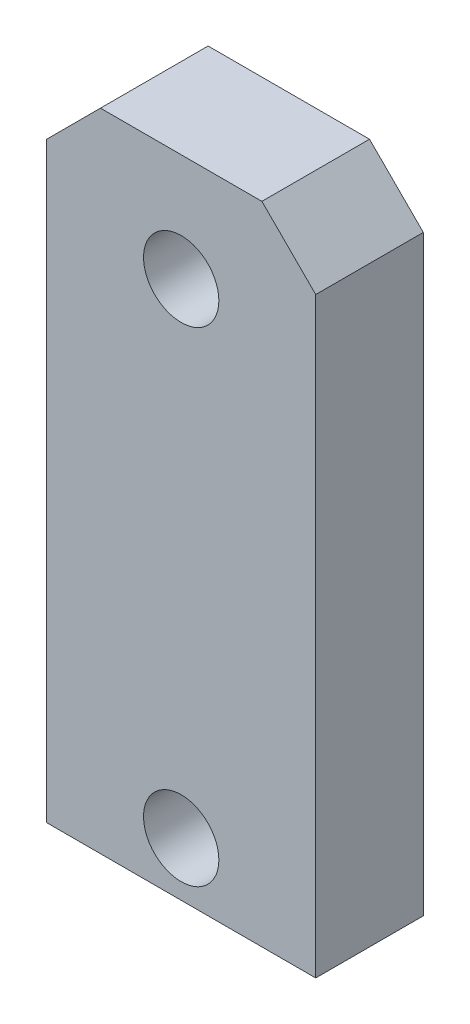
from build123d import *

# Parameters (mm, degrees)
SKETCH1_W           = 25
SKETCH1_H           = 60
BOSS_EXTRUDE1_DEPTH = 10
SKETCH2_R           = 3.5
CUT_EXTRUDE1_DEPTH  = 10
CHAMFER1_SIZE       = 5


with BuildPart() as part:
    # Sketch1 → Boss-Extrude1 (new body)
    with BuildSketch(Plane.XY):
        Rectangle(SKETCH1_W, SKETCH1_H)
    extrude(amount=BOSS_EXTRUDE1_DEPTH)

    # Sketch2 → Cut-Extrude1 (cut)
    with BuildSketch(Plane.XY.offset(10)):
        with Locations((0, 20)):
            Circle(SKETCH2_R)
        with Locations((0, -25)):
            Circle(SKETCH2_R)
    extrude(amount=-CUT_EXTRUDE1_DEPTH, mode=Mode.SUBTRACT)

    # Chamfer1
    chamfer1_edges = [part.edges().sort_by_distance(p)[0] for p in [
        (-12.5, 30, 5),
        (12.5, 30, 5),
    ]]
    chamfer(chamfer1_edges, length=CHAMFER1_SIZE)


solid = part.part
